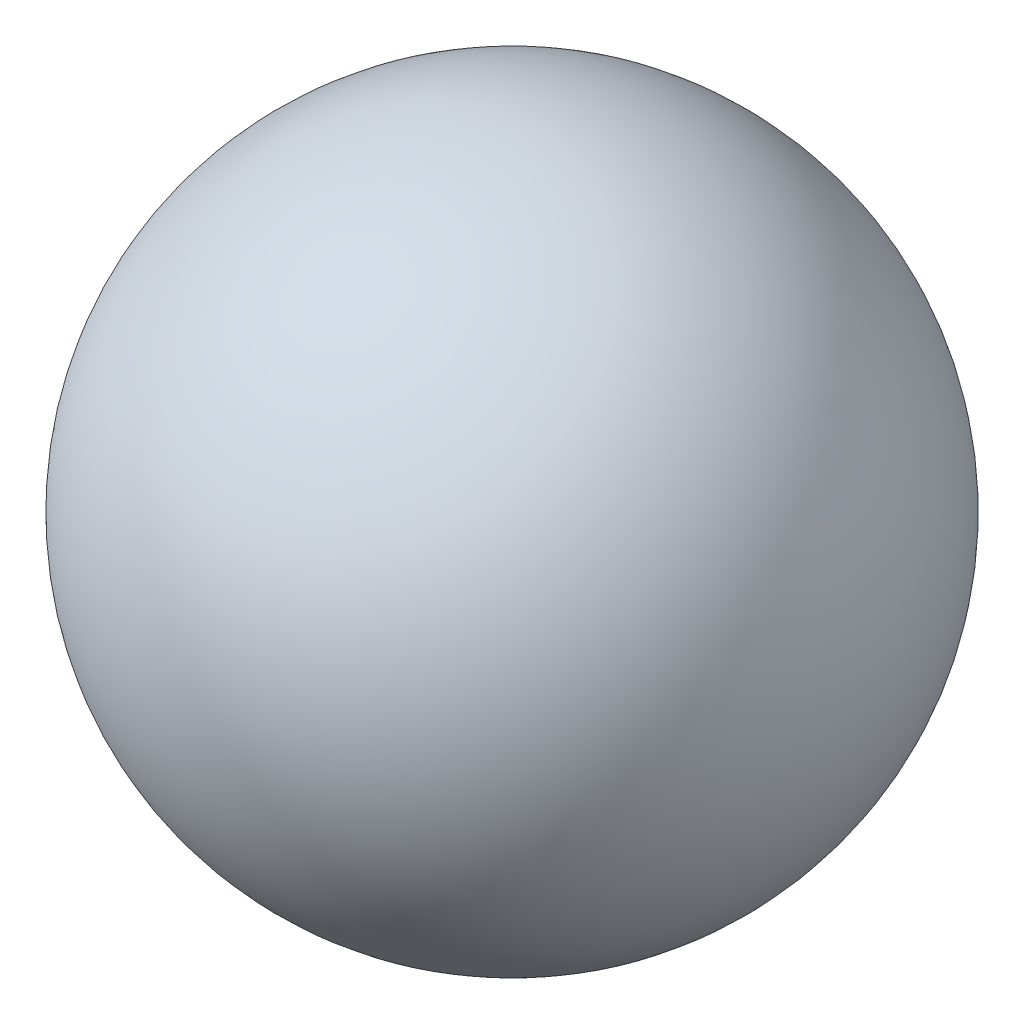
SolidWorks part; units mm, degrees
ref_plane "Front Plane" through (0, 0, 0) normal (0, 0, 1) x (1, 0, 0)
ref_plane "Top Plane" through (0, 0, 0) normal (0, 1, 0) x (1, 0, 0)
ref_plane "Right Plane" through (0, 0, 0) normal (1, 0, 0) x (0, 0, -1)
sketch "Sketch1" plane through (0, 0, 0) normal (0, 0, 1) x (1, 0, 0)
  line L0 (0, 25) -> (0, -25)
  arc A0 (0, -25) -> (0, 25) centre (0, 0) ccw
  dimension "D1" = 25
revolve "Revolve1" add sketch "Sketch1" angle 360 about L0
